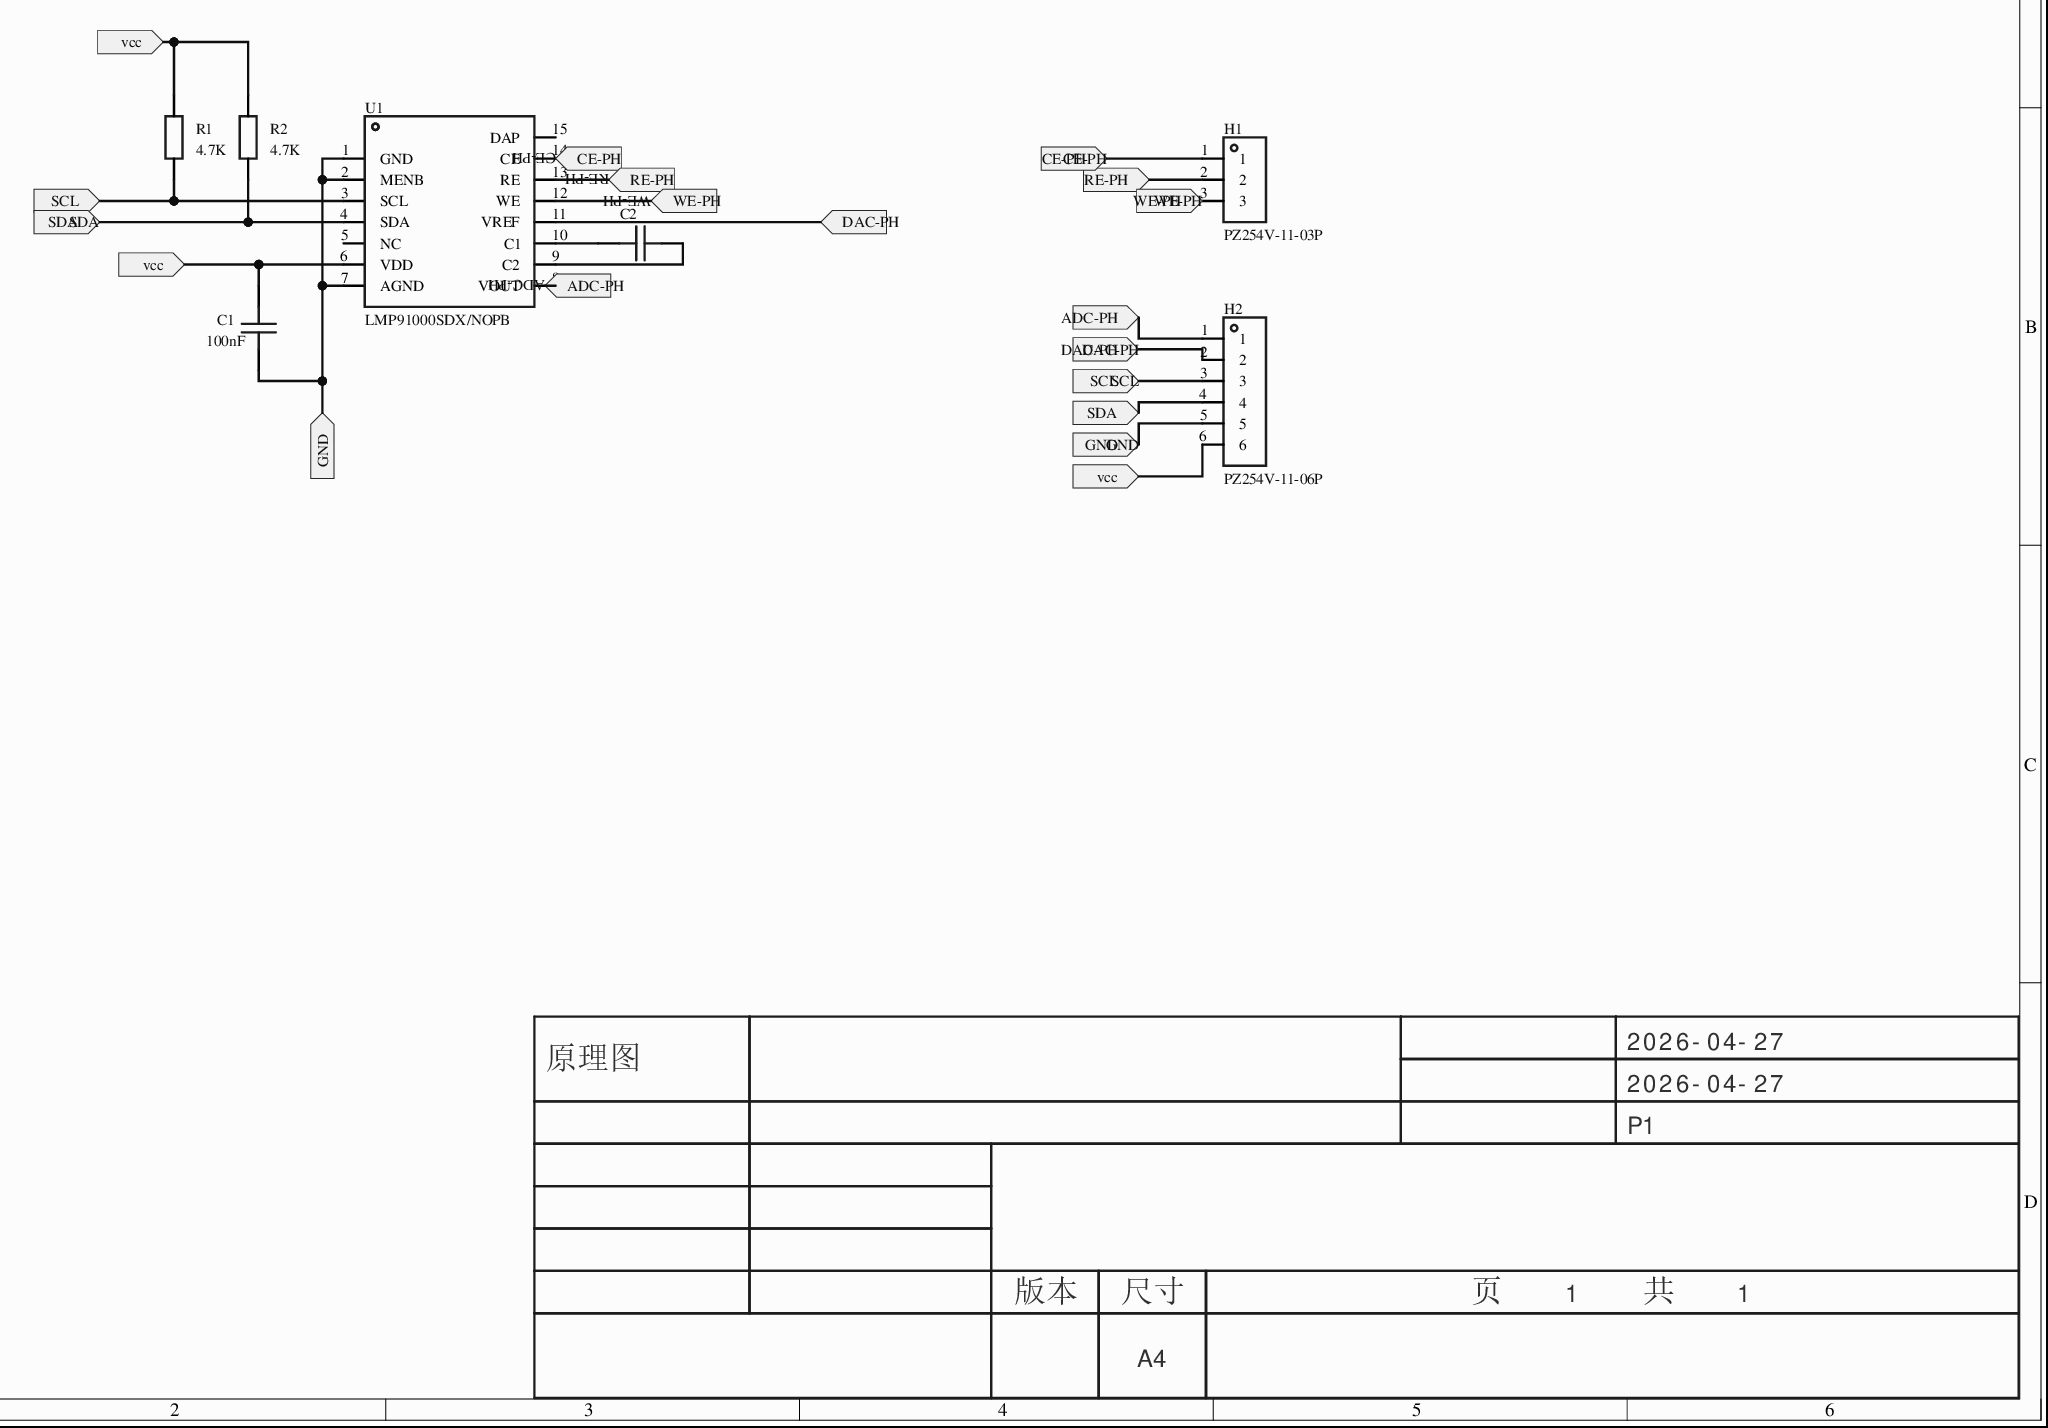
[diagram p0: MISC51980-2.schdoc]
# Altium project MISC51980.PrjPcb
1 sheet, 7 parts. Net scope: flat (ports and power ports of the same name join across sheets).
Board file: MISC51980.pcbdoc

## Sheet MISC51980-2.schdoc
size 297 x 209 mm; Version: V1.0; @Project Name: MISC51980; @Update Date: 2026-04-27; @Create Date: 2026-04-27; @Board Name: MISC51980; @Create Time: 13:08:49; @Page Count: 1; @Page No: 1; @Schematic Name: MISC51980; @Update Time: 13:08:49; Size: A4

### Parts
C1  100nF  [C0603]
C2  (no value)  [C0603]
H1  PZ254V-11-03P  [HDR-TH_3P-P2.54-V-M_PZ254V-11-03P]
H2  PZ254V-11-06P  [HDR-TH_6P-P2.54-V-M]
R1  4.7K  [R0603]
R2  4.7K  [R0603]
U1  LMP91000SDX/NOPB  [WSON-14_L4.0-W4.0-P0.50-BL-EP-1]

### Ports
ADC-PH (in), CE-PH (in), DAC-PH (in), GND (in), RE-PH (in), SCL (in), SDA (in), vcc (in), WE-PH (in)

### Nets
ADC-PH: H2.1 U1.8(VOUT) ; port ADC-PH
CE-PH: H1.1 U1.14(CE) ; port CE-PH
DAC-PH: H2.2 U1.11(VREF) ; port DAC-PH
GND: C1.2 H2.5 U1.1(GND) U1.2(MENB) U1.7(AGND) ; port GND
RE-PH: H1.2 U1.13(RE) ; port RE-PH
SCL: H2.3 R1.1 U1.3(SCL) ; port SCL
SDA: H2.4 R2.1 U1.4(SDA) ; port SDA
WE-PH: H1.3 U1.12(WE) ; port WE-PH
NetC1_1: C1.1 H2.6 R1.2 R2.2 U1.6(VDD) ; port vcc
NetC2_1: C2.1 U1.10(C1)
NetC2_2: C2.2 U1.9(C2)

Not connected (* = marked no-connect by the designer): U1 5(NC)* 15(DAP)*

### Notes on the sheet
- 2026-04-27
- 原理图
- P1
- 版本
- 尺寸
- A4
- 页    1    共    1

### Library data of the parts
C1 = CAP_0603: Symbol: Capacitance; ConvertToPcb: yes; ModelId: ac125912035d415993ca9572d50418b10819f05c4eef4c71ace90d822a990e87; ModelName: C0603_L1.6-W0.8-H0.8; ModelTransform: 62.992,31.496,0,0,0,0,0,0,0; Device: CAP_0603; AddInBom: yes; Supplier Footprint: 0603; FootprintName: C0603; Value: 100nF
C2 = CAP_0603: Symbol: Capacitance; Value: 2.2uF; ConvertToPcb: yes; ModelId: ac125912035d415993ca9572d50418b10819f05c4eef4c71ace90d822a990e87; ModelName: C0603_L1.6-W0.8-H0.8; ModelTransform: 62.992,31.496,0,0,0,0,0,0,0; Device: CAP_0603; AddInBom: yes; Supplier Footprint: 0603; FootprintName: C0603
H1 = PZ254V-11-03P: 插针结构:1x3P;间距:2.54mm;行距:-;圆针/方针:方针;安装方式:直插;排数:单排;总PIN位数:3P;额定电流:3A;额定电压:250V;配合针长度:6mm;塑高:2.5mm;端接针长度:3mm;工作温度:-40℃~+105℃;颜色:黑色;; Manufacturer: XFCN(兴飞); Symbol: PZ254V-11-03P_C2937625; AddInBom: yes; ModelId: bd28a638fbd247be9398fd5d39c366ec0819f05c4eef4c71ace90d822a990e87; ModelTransform: 300.3931,100,0,0,0,0,0,0,-118.11; Pin Structure: 1x3P; Pitch: 2.54mm; Circluar Pins/Square Pins: 方针; Current Rating: 3A; Voltage Rating (Max): 250V; Device: PZ254V-11-03P; LCSC Part Name: 1x3P 间距:2.54mm 方针 直插; SupplierPart: C2937625; ManufacturerPart: PZ254V-11-03P; Supplier Footprint: 插件,P=2.54mm; JLCPCB Part Class: Extended Part; Datasheet: https://item.szlcsc.com/datasheet/PZ254V-11-03P/3293280.html; Supplier: LCSC; ConvertToPcb: yes; FootprintName: HDR-TH_3P-P2.54-V-M_PZ254V-11-03P; ModelName: HDR-TH_3P-P2.54-V-M_PZ254V-11-03P; Row Spacing: -; Mounting Type: 直插; Number of Rows: 单排; Number of Pins: 3P; Length of Mating Pin: 6mm; Insulation Height: 2.5mm; Length of End Connection Pin: 3mm; Operating Temperature: -40℃~+105℃; Color: 黑色
H2 = PZ254V-11-06P: 插针结构:1x6P;间距:2.54mm;行距:-;圆针/方针:方针;安装方式:直插;排数:单排;总PIN位数:6P;额定电流:3A;额定电压:250V;配合针长度:6mm;塑高:2.5mm;端接针长度:3mm;触头材质:黄铜;触头镀层:-;工作温度:-40℃~+105℃;颜色:黑色;; Manufacturer: XFCN(兴飞); AddInBom: yes; ModelId: 66a147c6933d4029b68665bbcd1e29240819f05c4eef4c71ace90d822a990e87; ModelName: HDR-TH_6P-P2.54-M-LI-1X6P; ModelTransform: 590.1563,98.425,0,0,0,0,0,0,-118.11; Pin Structure: 1x6P; Pitch: 2.54mm; Circluar Pins/Square Pins: 方针; Current Rating: 3A; Voltage Rating (Max): 250V; Symbol: PZ254V-11-06P; Device: PZ254V-11-06P; LCSC Part Name: 1x6P 间距:2.54mm 方针 直插; SupplierPart: C492405; ManufacturerPart: PZ254V-11-06P; Supplier Footprint: 插件,P=2.54mm; JLCPCB Part Class: Extended Part; Datasheet: https://item.szlcsc.com/datasheet/PZ254V-11-06P/502961.html; Supplier: LCSC; ConvertToPcb: yes; FootprintName: HDR-TH_6P-P2.54-V-M; Row Spacing: -; Mounting Type: 直插; Number of Rows: 单排; Number of Pins: 6P; Length of Mating Pin: 6mm; Insulation Height: 2.5mm; Length of End Connection Pin: 3mm; Contact Material: 黄铜; Contact Plating: -; Operating Temperature: -40℃~+105℃; Color: 黑色
R1 R2 = Res_0603: Symbol: 电阻; 3D Model: fc143cca1e79419f9cd78b61e9279f080819f05c4eef4c71ace90d822a990e87; 3D Model Transform: 31.8897,63.7794,0,90,0,0,0,0,0; ConvertToPcb: yes; Device: Res_0603; Supplier Footprint: 0603; Value: 4.7K; AddInBom: yes; FootprintName: R0603; ModelName: R0603
U1 = LMP91000SDX/NOPB: 工作电压:2.7V~5.25V;工作电流:-;; Manufacturer: TI(德州仪器); AddInBom: yes; ModelId: 94ba79618d0446f0a31a118b8cb5c4850819f05c4eef4c71ace90d822a990e87; ModelName: WSON-14_L4.0-W4.0-H0.8-P0.50; ModelTransform: 157.48,158.268,0,90,0,0,0,0,0; Clock Frequency: 10kHz~100kHz; Voltage Reference Value: 2.5V; Quiescent Current (Iq): 0.85uA; Interface: I2C; Symbol: LMP91000SDX/NOPB; Device: LMP91000SDX/NOPB; LCSC Part Name: LMP91000传感器AFE系统; SupplierPart: C2651584; ManufacturerPart: LMP91000SDX/NOPB; Supplier Footprint: WSON-14(4x4); JLCPCB Part Class: Extended Part; Datasheet: https://www.ti.com/cn/lit/gpn/lmp91000; Supplier: LCSC; ConvertToPcb: yes; FootprintName: WSON-14_L4.0-W4.0-P0.50-BL-EP-1; Resolution(Bits): -; Gain Drift: -; Voltage - Supply: 2.7V~5.25V; Current - Supply: -; S/N Ratio: -; Operating Temperature: -40℃~+85℃; Data rate: -; Integral non - linearity: -; Sampling Rate: -; Voltage Reference Drift: -